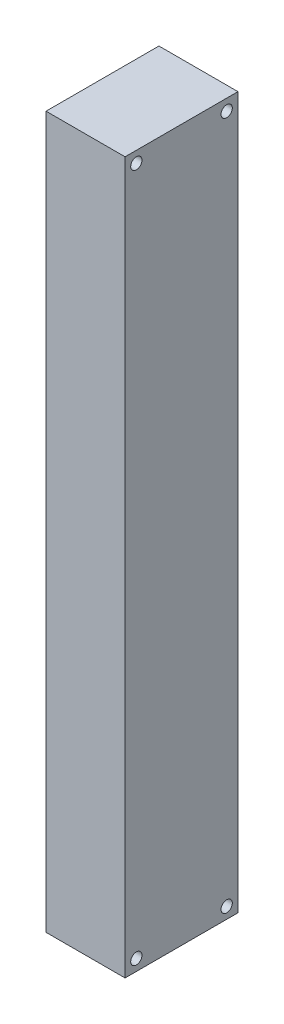
SolidWorks part; units mm, degrees
ref_plane "前视" through (0, 0, 0) normal (0, 0, 1) x (1, 0, 0)
ref_plane "上视" through (0, 0, 0) normal (0, 1, 0) x (1, 0, 0)
ref_plane "右视" through (0, 0, 0) normal (1, 0, 0) x (0, 0, -1)
sketch "草图1" plane through (0, 0, 0) normal (0, 0, 1) x (1, 0, 0)
  line L1 (0, 0) -> (35, 0)
  line L2 (0, 0) -> (0, 315)
  line L3 (0, 315) -> (35, 315)
  line L4 (35, 0) -> (35, 315)
  dimension "D1" = 315
  dimension "D2" = 35
extrude "凸台-拉伸1" add sketch "草图1" along normal blind 50
sketch "草图2" plane through (0, 0, 0) normal (-1, 0, 0) x (0, 0, 1)
  line L0 (50, 315) -> (50, 0) construction
  line L1 (50, 315) -> (0, 315) construction
  line L2 (0, 315) -> (0, 0) construction
  line L3 (50, 0) -> (0, 0) construction
  circle A0 centre (45, 310) radius 2.5
  circle A1 centre (5, 310) radius 2.5
  circle A2 centre (45, 5) radius 2.5
  circle A3 centre (5, 5) radius 2.5
  dimension "D1" = 5
  dimension "D2" = 5
  dimension "D7" = 5
  dimension "D8" = 5
  dimension "D9" = 5
  dimension "D10" = 5
  dimension "D11" = 5
  dimension "D12" = 5
  dimension "D3" = 5
  dimension "D4" = 5
  dimension "D5" = 5
  dimension "D6" = 5
extrude "切除-拉伸1" cut sketch "草图2" against normal blind 40
